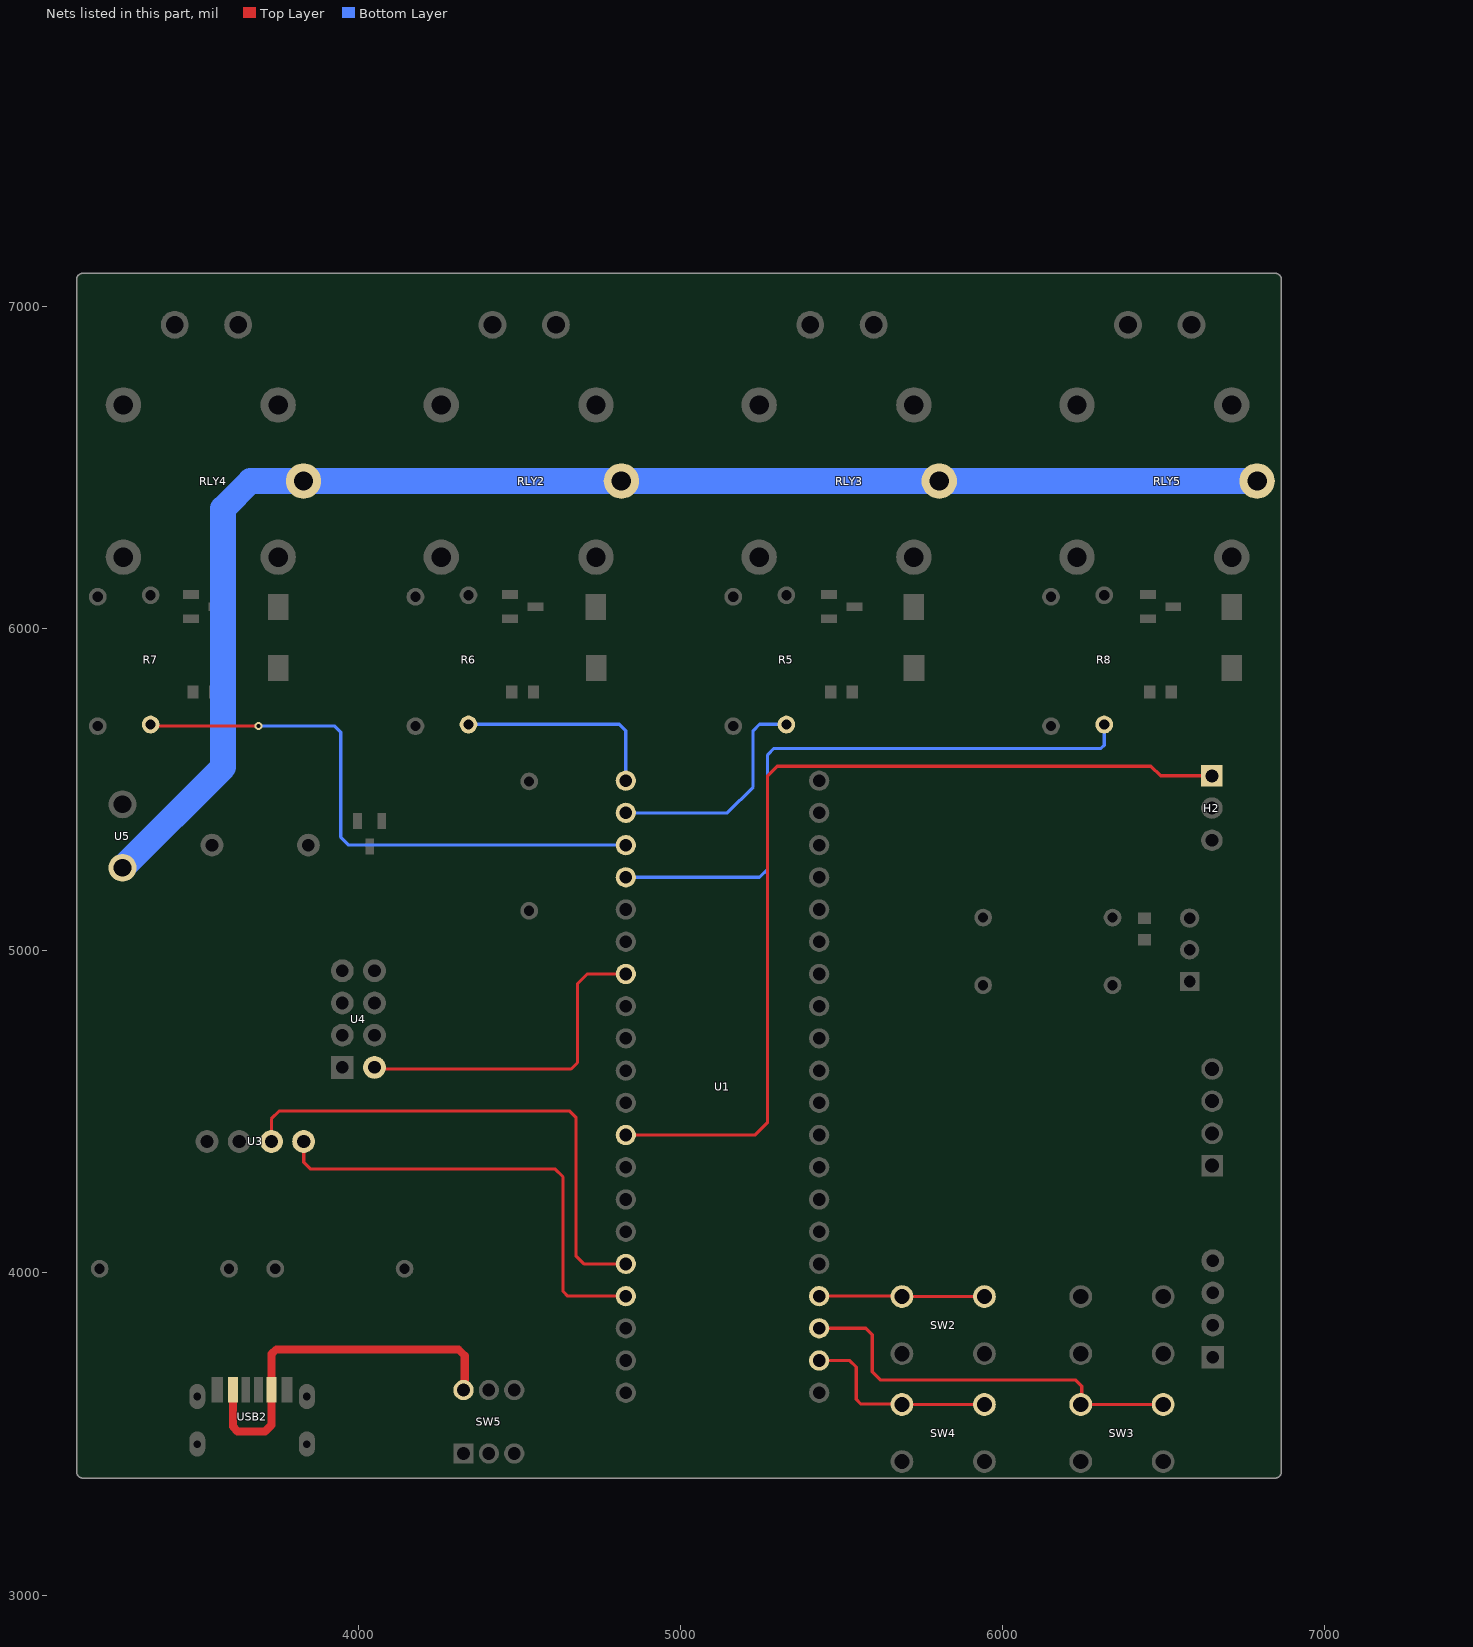
[diagram p0: the nets of this part, all layers, seen from the top]
# Altium PCB MISC62342.pcbdoc (part 2 of 2)
Units mil, origin at the board's own origin, x right, y up, seen from the top; angles counter-clockwise.
Board outline 3740 x 3740 mil, 2 copper layers (Top Layer, Bottom Layer), stack 62.206 mil thick; 50 components, 45 nets, 189 pads, 190 vias.

## Via types
v1: diameter 24.02, hole 12, Top Layer to Bottom Layer, 190 vias

## Nets (pads, with @x,y where several pads share a name; then routed paths per layer and width w, separated by ;. In a path a pad name is that pad's centre, name@x,y a point inside that pad or via, vN(x,y) a via of type N, cw(c..) or ccw(c..) an arc to the next point about the centre after c; other vN are vias at no path point) (continued)
PA10: U1.7 U4.5 | length 1047.8
  Top Layer w10: U4.5@4050,4638.19 4055,4633.19 4660,4633.19 4680,4653.19 4680,4898.19 4710,4928.19 U1.7@4830,4928.19
PB4: H2.1 U1.12 | length 2935.6
  Top Layer w10: U1.12@4830,4428.19 5230,4428.19 5270,4468.19 5270,5543.19 5300,5573.19 6460,5573.19 6490,5543.19 H2.1@6649.21,5543.19
PB8: U1.16 U3.3 | length 1629
  Top Layer w10: U3.3@3730,4408.19 3730,4478.19 3755,4503.19 4655,4503.19 4675,4483.19 4675,4053.19 4700,4028.18 U1.16@4830,4028.19
PB9: U1.17 U3.4 | length 1444.9
  Top Layer w10: U3.4@3830,4408.19 3830,4343.19 3850,4323.19 4610,4323.19 4635,4298.19 4635,3943.19 4650,3928.18 U1.17@4830,3928.19
PB12: R6.1 U1.1 | length 651.9
  Bottom Layer w10: R6.1@4341.67,5702.41 4342.46,5703.19 4810,5703.19 4830,5683.19 U1.1@4830,5528.19
PB13: R5.1 U1.2 | length 715.1
  Bottom Layer w10: U1.2@4830,5428.19 5145,5428.19 5225,5508.19 5225,5683.19 5245,5703.19 5327.54,5703.19 R5.1@5328.33,5702.41
PB14: R7.1 U1.3 | length 1820.4
  Top Layer w10: R7.1@3355,5702.41 3359.21,5698.19 v1(3690,5698.19)
  Bottom Layer w10: v1(3690,5698.19) 3925,5698.19 3945,5678.19 3945,5353.19 3970,5328.19 U1.3@4830,5328.19
PB15: R8.1 U1.4 | length 1927
  Bottom Layer w10: U1.4@4830,5228.19 5245,5228.19 5270,5253.19 5270,5608.19 5290,5628.19 6305,5628.19 6315,5638.19 R8.1@6315,5702.41
PC13: SW4.1 SW4.2 U1.22 | length 628
  Top Layer w10: U1.22@5430,3728.19 5525,3728.18 5545,3708.19 5545,3608.19 5560,3593.19 5665.63,3593.19 5667.05,3591.77 SW4.1@5687.05,3591.77 SW4.2@5942.95,3591.77
PC14: SW3.1 SW3.2 U1.23 | length 1270.5
  Top Layer w10: U1.23@5430,3828.19 5575,3828.18 5595,3808.19 5595,3693.19 5620,3668.19 6225,3668.19 6245,3648.19 6245,3594.72 SW3.1@6242.05,3591.77 SW3.2@6497.95,3591.77
PC15: SW2.1 SW2.2 U1.24 | length 513.5
  Top Layer w10: U1.24@5430,3928.19 5685.63,3928.18 SW2.1@5687.05,3926.77 SW2.2@5942.95,3926.77
VBUS: SW5.4 USB2.A9 USB2.B9 | length 1191.4
  Top Layer w25: USB2.B9@3610.16,3637.4 3610.16,3523.03 3625,3508.19 3710,3508.19 3730,3528.19 3730,3637.24 USB2.A9@3729.84,3637.4 3729.84,3748.03 3745,3763.19 4310,3763.19 4330,3743.19 4330,3640.35 SW5.4@4326.26,3636.62
VM: RLY2.5 RLY3.5 RLY4.5 RLY5.5 U5.2 | length 4489.5
  Bottom Layer w80: U5.2@3267.64,5257.86 3580,5570.22 3580,6373.19 3665,6458.19 RLY4.5@3829.53,6458.19 RLY2.5@4816.19,6458.19 RLY3.5@5802.86,6458.19 RLY5.5@6789.53,6458.19
pads on no net: H3.2 RLY2.3 RLY3.3 RLY4.3 RLY5.3 SW5.1 SW5.2 SW5.3 SW5.6 U1.8 U1.9 U1.10 U1.11 U1.13 U1.14 U1.15 U1.21 U1.30 U1.31 U1.32 U1.33 U1.34 U1.35 U1.36 U1.37 U4.2 U4.3 U4.6 U4.7
copper on no net:
  other v1: 3925,7773.19

## Polygon pours and split planes (outlines as drawn)
GND on Top Layer (solid, remove dead copper, pour order 0): 3055,7168.19 3055,3253.19 7025,3253.19 7025,7168.19
GND on Bottom Layer (solid, remove dead copper, pour order 2): 3000,7263.19 3000,3271.35 6985.25,3271.35 6985.25,7263.19

## Keep-outs
Board Outline Layer:
  region: 3130,5103.19 3130,4493.19 3460,4493.19 3460,5103.19
  region: 3136.57,6765.27 3136.57,6151.1 3892.49,6151.1 3892.49,6765.27
  region: 4123.24,6765.27 4123.24,6151.1 4879.15,6151.1 4879.15,6765.27
  region: 5109.9,6765.27 5109.9,6151.1 5865.82,6151.1 5865.82,6765.27
  region: 6096.57,6765.27 6096.57,6151.1 6852.49,6151.1 6852.49,6765.27
  lines w10: 3125,3383.19 3125,7083.19 cw(c3145,7083.19) 3145,7103.19 6845,7103.19 cw(c6845,7083.19) 6865,7083.19 6865,3383.19 cw(c6845,3383.19) 6845,3363.19 3145,3363.19 cw(c3145,3383.19) 3125,3383.19

## Other copper
Top Layer:
  region net +5V: 5736.99,5800.76 5711.99,5800.76 5711.68,5806.18 5710.74,5811.53 5709.19,5816.73 5707.04,5821.72 5704.34,5826.43 5701.11,5830.79 5697.39,5834.75 5693.24,5838.26 5755.74,5838.26 5751.59,5834.75 5747.88,5830.79 5744.65,5826.43 5741.94,5821.72 5739.8,5816.73 5738.25,5811.53 5737.31,5806.18 5736.99,5800.76
  region net +5V: 5793.88,5891.04 5793.88,5866.04 5788.46,5865.73 5783.11,5864.79 5777.91,5863.24 5772.92,5861.09 5768.21,5858.39 5763.85,5855.16 5759.89,5851.44 5756.38,5847.29 5756.38,5909.79 5759.89,5905.64 5763.85,5901.93 5768.21,5898.7 5772.92,5895.99 5777.91,5893.85 5783.11,5892.3 5788.46,5891.36 5793.88,5891.04
  region net +5V: 5655.1,5866.04 5655.1,5891.04 5660.52,5891.36 5665.87,5892.3 5671.08,5893.85 5676.07,5895.99 5680.77,5898.7 5685.14,5901.93 5689.1,5905.64 5692.6,5909.79 5692.6,5847.29 5689.1,5851.44 5685.14,5855.16 5680.77,5858.39 5676.07,5861.09 5671.08,5863.24 5665.87,5864.79 5660.52,5865.73 5655.1,5866.04
  region net +5V: 4773.69,5932.08 4782.97,5906.01 4779.02,5900.11 4775.72,5893.81 4773.12,5887.2 4771.23,5880.35 4770.1,5873.33 4769.72,5866.24 4733.91,5918.82 4741.01,5919.21 4748.03,5920.34 4754.88,5922.23 4761.49,5924.83 4767.78,5928.13 4773.69,5932.08
  region net +5V: 4807.22,5890.69 4807.22,5865.69 4801.79,5865.37 4796.45,5864.43 4791.24,5862.88 4786.25,5860.74 4781.54,5858.03 4777.18,5854.8 4773.22,5851.09 4769.72,5846.94 4769.72,5909.44 4773.22,5905.29 4777.18,5901.57 4781.54,5898.34 4786.25,5895.64 4791.24,5893.49 4796.45,5891.94 4801.79,5891 4807.22,5890.69
  region net +5V: 4752.5,5800.76 4727.5,5800.76 4727.19,5806.18 4726.25,5811.53 4724.69,5816.73 4722.55,5821.72 4719.85,5826.43 4716.61,5830.79 4712.9,5834.75 4708.75,5838.26 4769.72,5838.26 4765.36,5834.02 4761.56,5829.28 4758.36,5824.11 4755.83,5818.59 4753.99,5812.8 4752.87,5806.82 4752.5,5800.76
  region net +5V: 3762.5,5800.76 3737.5,5800.76 3737.1,5806.91 3735.91,5812.95 3733.96,5818.79 3731.26,5824.33 3727.88,5829.48 3723.86,5834.15 3719.27,5838.26 3781.25,5838.26 3777.1,5834.75 3773.39,5830.79 3770.15,5826.43 3767.45,5821.72 3765.31,5816.73 3763.75,5811.53 3762.81,5806.18 3762.5,5800.76
  region net +5V: 3820.55,5885.69 3820.55,5860.69 3815.13,5860.37 3809.78,5859.43 3804.58,5857.88 3799.59,5855.74 3794.88,5853.03 3790.51,5849.8 3786.55,5846.09 3783.05,5841.94 3783.05,5904.44 3786.55,5900.29 3790.51,5896.57 3794.88,5893.34 3799.59,5890.64 3804.58,5888.49 3809.78,5886.94 3815.13,5886 3820.55,5885.69
  region net +5V: 3787.02,5932.08 3796.31,5906.01 3792.35,5900.11 3789.06,5893.81 3786.45,5887.2 3784.57,5880.35 3783.43,5873.33 3783.05,5866.24 3747.25,5918.82 3754.34,5919.21 3761.36,5920.34 3768.21,5922.23 3774.82,5924.83 3781.12,5928.13 3787.02,5932.08
  region net +5V: 6756.31,5851.07 6747.02,5825 6741.12,5828.95 6734.82,5832.25 6728.21,5834.86 6721.36,5836.74 6714.34,5837.88 6707.25,5838.26 6743.05,5890.85 6743.43,5883.75 6744.57,5876.74 6746.45,5869.88 6749.06,5863.27 6752.35,5856.98 6756.31,5851.07
  region net +5V: 6747.02,5932.08 6756.31,5906.01 6752.35,5900.11 6749.06,5893.81 6746.45,5887.2 6744.57,5880.35 6743.43,5873.33 6743.05,5866.24 6707.25,5918.82 6714.34,5919.21 6721.36,5920.34 6728.21,5922.23 6734.82,5924.83 6741.12,5928.13 6747.02,5932.08
  region net PB4: 6600.75,5538.19 6600.75,5548.19 6604.2,5548.51 6607.54,5549.46 6610.65,5551.02 6613.42,5553.11 6615.75,5555.69 6615.75,5530.69 6613.42,5533.26 6610.65,5535.36 6607.54,5536.91 6604.2,5537.87 6600.75,5538.19
  region net +5V: 6694.77,5455.69 6694.77,5430.69 6691.32,5430.4 6688.1,5429.6 6685.06,5428.36 6682.17,5426.75 6679.39,5424.84 6676.68,5422.71 6671.35,5418.09 6671.35,5468.29 6676.68,5463.66 6679.39,5461.53 6682.17,5459.62 6685.06,5458.01 6688.1,5456.77 6691.32,5455.97
  region net +3.3V: 6645,4682.25 6665,4674.75 6665.08,4672.6 6665.29,4670.68 6665.65,4668.96 6666.13,4667.41 6666.72,4666 6667.42,4664.7 6669.1,4662.31 6673.3,4657.57 6675.68,4654.75 6678.12,4651.32 6628.49,4658.82 6634.55,4663.89 6637.34,4666.44 6639.84,4669.09 6641.95,4671.93 6642.83,4673.44 6643.58,4675.02 6644.18,4676.68 6644.63,4678.43 6644.91,4680.29
  region net +3.3V: 6691.56,4648.19 6699.06,4628.19 6697.1,4628.09 6695.25,4627.82 6693.49,4627.37 6691.83,4626.77 6690.25,4626.02 6688.74,4625.14 6685.91,4623.03 6683.25,4620.53 6680.7,4617.74 6675.64,4611.68 6668.14,4661.31 6671.57,4658.86 6674.39,4656.49 6679.12,4652.29 6681.51,4650.61 6682.81,4649.91 6684.22,4649.31 6685.78,4648.84 6687.5,4648.48 6689.41,4648.26
  region net +5V: 4189.52,5659.88 4164.52,5659.88 4164.33,5662.29 4163.81,5664.85 4163.01,5667.47 4161.96,5670.1 4160.73,5672.66 4159.35,5675.07 4157.87,5677.26 4156.35,5679.17 4197.69,5679.17 4196.16,5677.26 4194.69,5675.07 4193.31,5672.66 4192.07,5670.1 4191.02,5667.47 4190.22,5664.85 4189.7,5662.29
  region net +5V: 4139.5,5684.9 4139.5,5709.9 4141.91,5710.08 4144.46,5710.6 4147.09,5711.4 4149.72,5712.45 4152.28,5713.69 4154.69,5715.07 4156.88,5716.54 4158.79,5718.07 4158.79,5676.73 4156.88,5678.25 4154.69,5679.73 4152.28,5681.11 4149.72,5682.34 4147.09,5683.39 4144.46,5684.19 4141.91,5684.71
  region net +5V: 5198.74,5679.71 5181.06,5662.03 5179.23,5663.6 5177.05,5665.04 5174.62,5666.33 5172.03,5667.45 5169.34,5668.39 5166.66,5669.11 5164.07,5669.62 5161.64,5669.89 5190.87,5699.12 5191.14,5696.7 5191.65,5694.1 5192.38,5691.42 5193.31,5688.74 5194.43,5686.14 5195.72,5683.71 5197.16,5681.54
  region net +5V: 5125.85,5684.9 5125.85,5709.9 5128.26,5710.08 5130.82,5710.6 5133.45,5711.4 5136.07,5712.45 5138.63,5713.69 5141.04,5715.07 5143.23,5716.54 5145.14,5718.07 5145.14,5676.73 5143.23,5678.25 5141.04,5679.73 5138.63,5681.11 5136.07,5682.34 5133.45,5683.39 5130.82,5684.19 5128.26,5684.71
  region net +5V: 3203.16,5659.88 3178.16,5659.88 3177.98,5662.29 3177.46,5664.85 3176.66,5667.47 3175.61,5670.1 3174.37,5672.66 3172.99,5675.07 3171.52,5677.26 3169.99,5679.17 3211.33,5679.17 3209.81,5677.26 3208.33,5675.07 3206.95,5672.66 3205.72,5670.1 3204.67,5667.47 3203.87,5664.85 3203.35,5662.29
  region net +5V: 6115.57,5680.69 6109.26,5705.69 6111.67,5705.9 6114.29,5706.49 6117.01,5707.41 6119.72,5708.61 6122.34,5710.03 6124.75,5711.61 6126.85,5713.29 6128.55,5715.04 6134.86,5674.19 6130.56,5676.57 6128.12,5677.67 6125.57,5678.66 6122.99,5679.49 6120.42,5680.13 6117.92,5680.54
  region net PA8: 4567.52,5129.25 4567.52,5119.25 4565.45,5119.16 4563.65,5118.9 4562.1,5118.47 4560.76,5117.9 4559.59,5117.19 4558.55,5116.36 4556.76,5114.35 4553.32,5109.33 4551.12,5106.5 4549.78,5105.05 4548.23,5103.58 4548.23,5144.92 4549.78,5143.45 4551.12,5141.99 4553.32,5139.16 4556.76,5134.14 4558.55,5132.14 4559.59,5131.3 4560.76,5130.59 4562.1,5130.02 4563.65,5129.6 4565.45,5129.34
  region net PA3: 6350,4859.04 6340,4852.72 6339.9,4854.67 6339.62,4856.41 6339.17,4857.98 6338.55,4859.38 6337.79,4860.64 6336.89,4861.8 6334.73,4863.85 6332.18,4865.72 6329.34,4867.58 6326.29,4869.62 6323.15,4872.01 6364,4878.33 6362.39,4876.2 6360.34,4873.92 6355.69,4869.07 6353.51,4866.55 6351.7,4864.02 6350.99,4862.76 6350.46,4861.51 6350.12,4860.27
  region net PA3: 6378.31,4898.19 6378.31,4888.19 6376.24,4888.1 6374.44,4887.84 6372.89,4887.41 6371.55,4886.84 6370.38,4886.13 6369.34,4885.29 6367.55,4883.29 6364.11,4878.27 6361.91,4875.44 6360.57,4873.98 6359.02,4872.52 6359.02,4913.86 6360.57,4912.39 6361.91,4910.93 6364.11,4908.1 6367.55,4903.08 6369.34,4901.08 6370.38,4900.24 6371.55,4899.53 6372.89,4898.96 6374.44,4898.54 6376.24,4898.28
  region net +3.3V: 5929.21,4930.71 5949.21,4930.71 5949.45,4927.81 5950.13,4925.14 5951.18,4922.65 5952.54,4920.31 5954.16,4918.05 5955.96,4915.85 5959.88,4911.42 5918.54,4911.42 5922.46,4915.85 5924.26,4918.05 5925.88,4920.31 5927.24,4922.65 5928.29,4925.14 5928.97,4927.81
  region net +3.3V: 5949.21,5065.67 5929.21,5065.67 5928.97,5068.56 5928.29,5071.23 5927.24,5073.72 5925.88,5076.07 5924.26,5078.32 5922.46,5080.53 5918.54,5084.96 5959.88,5084.96 5955.96,5080.53 5954.16,5078.32 5952.54,5076.07 5951.18,5073.72 5950.13,5071.23 5949.45,5068.56
  region net +5V: 4800.06,6230.81 4821.52,6173.98 4819.01,6176.32 4816.32,6178.47 4813.49,6180.41 4810.53,6182.14 4807.47,6183.65 4804.32,6184.9 4801.12,6185.89 4797.89,6186.61 4794.65,6187.03 4791.42,6187.15 4788.23,6186.94 4785.1,6186.4 4782.05,6185.5 4779.11,6184.23 4776.29,6182.59 4773.63,6180.54 4774.74,6262.4 4779.52,6257.69 4782.96,6253.69 4785.52,6250.15 4787.61,6246.82 4789.68,6243.47 4792.16,6239.85 4795.47,6235.71
  region net +5V: 5798.08,6235.69 5799.91,6210.69 5796.11,6210.52 5792.73,6210.03 5789.72,6209.25 5787.04,6208.18 5784.63,6206.86 5782.44,6205.31 5780.42,6203.54 5778.52,6201.58 5774.87,6197.16 5771.07,6192.24 5766.72,6186.97 5764.21,6184.26 5761.41,6181.53 5759.58,6264.01 5762.54,6261.36 5765.15,6258.73 5769.59,6253.61 5773.35,6248.83 5776.89,6244.54 5778.72,6242.63 5780.67,6240.92 5782.8,6239.4 5785.16,6238.12 5787.81,6237.09 5790.81,6236.32 5794.21,6235.85
  region net +5V: 3825.67,6234.47 3825.67,6209.47 3821.83,6209.3 3818.44,6208.82 3815.44,6208.05 3812.78,6207 3810.39,6205.7 3808.23,6204.16 3806.25,6202.42 3804.38,6200.48 3800.78,6196.13 3797.01,6191.27 3792.61,6186.08 3790.05,6183.41 3787.17,6180.72 3787.17,6263.22 3790.05,6260.53 3792.61,6257.86 3797.01,6252.66 3800.78,6247.8 3804.38,6243.45 3806.25,6241.52 3808.23,6239.77 3810.39,6238.24 3812.78,6236.94 3815.44,6235.89 3818.44,6235.11 3821.83,6234.63
  region net +5V: 6774.23,6196.64 6771.87,6163.64 6769.27,6165.98 6766.58,6167.9 6763.81,6169.44 6760.97,6170.63 6758.04,6171.49 6755.04,6172.06 6751.98,6172.37 6748.85,6172.44 6745.65,6172.3 6742.4,6171.99 6735.74,6170.96 6721.88,6168.1 6762.85,6239.71 6763.55,6237.34 6764.15,6234.78 6765.09,6229.17 6766.71,6217.03 6767.76,6211.04 6768.43,6208.19 6769.24,6205.47 6770.19,6202.92 6771.33,6200.57 6772.66,6198.47
  region net PA0: 6237.05,3975.01 6247.05,3975.01 6247.17,3972.18 6247.53,3969.76 6248.12,3967.71 6248.9,3965.97 6249.88,3964.49 6251.03,3963.22 6252.34,3962.1 6253.79,3961.08 6260.7,3956.95 6262.63,3955.64 6264.6,3954.11 6266.6,3952.32 6268.62,3950.2 6215.48,3950.2 6217.5,3952.32 6219.5,3954.11 6221.47,3955.64 6223.4,3956.95 6230.31,3961.08 6231.76,3962.1 6233.07,3963.22 6234.22,3964.49 6235.2,3965.97 6235.98,3967.71 6236.57,3969.76 6236.93,3972.18
  region net PA0: 6290.29,3931.77 6290.29,3921.77 6287.46,3921.64 6285.04,3921.28 6282.99,3920.7 6281.25,3919.91 6279.77,3918.94 6278.5,3917.78 6277.38,3916.48 6276.36,3915.02 6272.23,3908.11 6270.92,3906.19 6269.4,3904.22 6267.6,3902.21 6265.49,3900.19 6265.49,3953.34 6267.6,3951.32 6269.4,3949.32 6270.92,3947.34 6272.23,3945.42 6276.36,3938.51 6277.38,3937.06 6278.5,3935.75 6279.77,3934.6 6281.25,3933.62 6282.99,3932.83 6285.04,3932.25 6287.46,3931.89
  region net PA0: 6449.71,3921.77 6449.71,3931.77 6452.54,3931.89 6454.96,3932.25 6457.01,3932.83 6458.75,3933.62 6460.23,3934.6 6461.5,3935.75 6462.62,3937.06 6463.64,3938.51 6467.77,3945.42 6469.08,3947.34 6470.6,3949.32 6472.4,3951.32 6474.51,3953.34 6474.51,3900.19 6472.4,3902.21 6470.6,3904.22 6469.08,3906.19 6467.77,3908.11 6463.64,3915.02 6462.62,3916.48 6461.5,3917.78 6460.23,3918.94 6458.75,3919.91 6457.01,3920.7 6454.96,3921.28 6452.54,3921.64
  region net PC15: 5637.77,3923.18 5639.89,3933.18 5641.48,3933.36 5643.09,3933.87 5644.73,3934.68 5646.38,3935.74 5649.7,3938.46 5653,3941.75 5659.26,3948.74 5662.11,3951.84 5664.7,3954.26 5662.57,3901.15 5660.57,3903.21 5658.85,3905.26 5656.07,3909.24 5653.86,3912.96 5651.82,3916.3 5650.75,3917.78 5649.58,3919.12 5648.26,3920.29 5646.75,3921.29 5644.99,3922.1 5642.94,3922.69 5640.55,3923.06
  region net PC15: 5735.29,3931.77 5735.29,3921.77 5732.46,3921.64 5730.04,3921.28 5727.99,3920.7 5726.25,3919.91 5724.77,3918.94 5723.5,3917.78 5722.38,3916.48 5721.36,3915.02 5717.23,3908.11 5715.92,3906.19 5714.4,3904.22 5712.6,3902.21 5710.49,3900.19 5710.49,3953.34 5712.6,3951.32 5714.4,3949.32 5715.92,3947.34 5717.23,3945.42 5721.36,3938.51 5722.38,3937.06 5723.5,3935.75 5724.77,3934.6 5726.25,3933.62 5727.99,3932.83 5730.04,3932.25 5732.46,3931.89
  region net PC15: 5894.71,3921.77 5894.71,3931.77 5897.54,3931.89 5899.96,3932.25 5902.01,3932.83 5903.75,3933.62 5905.23,3934.6 5906.5,3935.75 5907.62,3937.06 5908.64,3938.51 5912.77,3945.42 5914.08,3947.34 5915.6,3949.32 5917.4,3951.32 5919.51,3953.34 5919.51,3900.19 5917.4,3902.21 5915.6,3904.22 5914.08,3906.19 5912.77,3908.11 5908.64,3915.02 5907.62,3916.48 5906.5,3917.78 5905.23,3918.94 5903.75,3919.91 5902.01,3920.7 5899.96,3921.28 5897.54,3921.64
  region net PC14: 6240,3642.14 6250,3637.71 6250.17,3636.1 6250.67,3634.47 6251.45,3632.83 6252.48,3631.19 6255.13,3627.91 6258.32,3624.68 6265.12,3618.48 6268.13,3615.6 6270.48,3612.91 6217.52,3617.33 6219.62,3619.22 6221.71,3620.86 6225.77,3623.57 6229.57,3625.81 6232.97,3627.94 6234.49,3629.06 6235.85,3630.29 6237.05,3631.65 6238.07,3633.21 6238.89,3634.99 6239.5,3637.04 6239.87,3639.41
  region net PC14: 6290.29,3596.77 6290.29,3586.77 6287.46,3586.64 6285.04,3586.28 6282.99,3585.7 6281.25,3584.91 6279.77,3583.94 6278.5,3582.78 6277.38,3581.48 6276.36,3580.02 6272.23,3573.11 6270.92,3571.19 6269.4,3569.22 6267.6,3567.21 6265.49,3565.19 6265.49,3618.34 6267.6,3616.32 6269.4,3614.32 6270.92,3612.34 6272.23,3610.42 6276.36,3603.51 6277.38,3602.06 6278.5,3600.75 6279.77,3599.6 6281.25,3598.62 6282.99,3597.83 6285.04,3597.25 6287.46,3596.89
  region net PC14: 6449.71,3586.77 6449.71,3596.77 6452.54,3596.89 6454.96,3597.25 6457.01,3597.83 6458.75,3598.62 6460.23,3599.6 6461.5,3600.75 6462.62,3602.06 6463.64,3603.51 6467.77,3610.42 6469.08,3612.34 6470.6,3614.32 6472.4,3616.32 6474.51,3618.34 6474.51,3565.19 6472.4,3567.21 6470.6,3569.22 6469.08,3571.19 6467.77,3573.11 6463.64,3580.02 6462.62,3581.48 6461.5,3582.78 6460.23,3583.94 6458.75,3584.91 6457.01,3585.7 6454.96,3586.28 6452.54,3586.64
  region net PC13: 5735.29,3596.77 5735.29,3586.77 5732.46,3586.64 5730.04,3586.28 5727.99,3585.7 5726.25,3584.91 5724.77,3583.94 5723.5,3582.78 5722.38,3581.48 5721.36,3580.02 5717.23,3573.11 5715.92,3571.19 5714.4,3569.22 5712.6,3567.21 5710.49,3565.19 5710.49,3618.34 5712.6,3616.32 5714.4,3614.32 5715.92,3612.34 5717.23,3610.42 5721.36,3603.51 5722.38,3602.06 5723.5,3600.75 5724.77,3599.6 5726.25,3598.62 5727.99,3597.83 5730.04,3597.25 5732.46,3596.89
  region net PC13: 5637.76,3588.19 5639.89,3598.19 5641.48,3598.37 5643.09,3598.88 5644.73,3599.68 5646.38,3600.74 5649.7,3603.47 5653,3606.75 5659.26,3613.74 5662.11,3616.84 5664.7,3619.26 5662.57,3566.15 5660.56,3568.22 5658.85,3570.26 5656.07,3574.24 5653.86,3577.97 5651.82,3581.3 5650.75,3582.78 5649.58,3584.12 5648.26,3585.3 5646.75,3586.29 5644.99,3587.1 5642.93,3587.69 5640.54,3588.06
  region net PC13: 5894.71,3586.77 5894.71,3596.77 5897.54,3596.89 5899.96,3597.25 5902.01,3597.83 5903.75,3598.62 5905.23,3599.6 5906.5,3600.75 5907.62,3602.06 5908.64,3603.51 5912.77,3610.42 5914.08,3612.34 5915.6,3614.32 5917.4,3616.32 5919.51,3618.34 5919.51,3565.19 5917.4,3567.21 5915.6,3569.22 5914.08,3571.19 5912.77,3573.11 5908.64,3580.02 5907.62,3581.48 5906.5,3582.78 5905.23,3583.94 5903.75,3584.91 5902.01,3585.7 5899.96,3586.28 5897.54,3586.64
  region net VBUS: 4317.5,3682.15 4342.5,3676.54 4342.72,3673.43 4343.33,3670.48 4344.29,3667.67 4345.53,3664.95 4346.99,3662.31 4348.63,3659.7 4352.19,3654.49 4305.28,3660.1 4307.56,3662.28 4309.77,3664.7 4311.83,3667.31 4313.68,3670.1 4315.24,3673.01 4316.45,3676.01 4317.23,3679.07
  region net +5V: 4392.5,3679.49 4417.5,3679.49 4417.75,3676.39 4418.46,3673.39 4419.56,3670.48 4420.98,3667.68 4422.66,3664.97 4424.54,3662.37 4428.62,3657.44 4381.38,3657.44 4385.46,3662.37 4387.34,3664.97 4389.03,3667.68 4390.45,3670.48 4391.55,3673.39 4392.25,3676.39
  region net PA2: 6603.73,3933.19 6603.73,3943.19 6606.56,3943.31 6608.98,3943.67 6611.03,3944.25 6612.76,3945.04 6614.24,3946.02 6615.52,3947.17 6616.64,3948.48 6617.66,3949.93 6621.79,3956.84 6623.1,3958.76 6624.62,3960.74 6626.42,3962.74 6628.53,3964.76 6628.53,3911.61 6626.42,3913.63 6624.62,3915.64 6623.1,3917.61 6621.79,3919.53 6617.66,3926.44 6616.64,3927.9 6615.52,3929.2 6614.24,3930.36 6612.76,3931.33 6611.03,3932.12 6608.98,3932.7 6606.56,3933.06
  region net +3.3V: 6717.4,3748.19 6717.4,3728.19 6712.45,3727.86 6707.58,3726.88 6702.89,3725.26 6698.45,3723.04 6694.34,3720.26 6690.64,3716.95 6687.4,3713.19 6687.4,3763.19 6690.64,3759.42 6694.34,3756.12 6698.45,3753.33 6702.89,3751.11 6707.58,3749.5 6712.45,3748.52 6717.4,3748.19
  region net +3.3V: 3625,4459.94 3645,4452.44 3645.08,4450.09 3645.33,4448.01 3645.72,4446.16 3646.26,4444.52 3646.92,4443.03 3647.7,4441.68 3649.57,4439.22 3654.25,4434.34 3656.89,4431.35 3659.62,4427.64 3607,4435.14 3613.61,4440.59 3616.65,4443.24 3619.37,4445.98 3621.68,4448.92 3622.64,4450.49 3623.45,4452.15 3624.11,4453.92 3624.6,4455.79 3624.9,4457.8
  region net PB8: 3725,4456.43 3735,4456.43 3735.12,4453.6 3735.48,4451.18 3736.07,4449.13 3736.85,4447.39 3737.83,4445.91 3738.98,4444.64 3740.29,4443.52 3741.74,4442.5 3748.65,4438.37 3750.58,4437.06 3752.55,4435.53 3754.55,4433.74 3756.57,4431.62 3703.43,4431.62 3705.45,4433.74 3707.45,4435.53 3709.42,4437.06 3711.35,4438.37 3718.26,4442.5 3719.71,4443.52 3721.02,4444.64 3722.17,4445.91 3723.15,4447.39 3723.93,4449.13 3724.52,4451.18 3724.88,4453.6
  region net PB9: 3835,4359.95 3825,4359.95 3824.88,4362.78 3824.52,4365.19 3823.93,4367.24 3823.15,4368.98 3822.17,4370.46 3821.02,4371.74 3819.71,4372.86 3818.26,4373.88 3811.35,4378.01 3809.42,4379.32 3807.45,4380.84 3805.45,4382.64 3803.43,4384.75 3856.57,4384.75 3854.55,4382.64 3852.55,4380.84 3850.58,4379.32 3848.65,4378.01 3841.74,4373.88 3840.29,4372.86 3838.98,4371.74 3837.83,4370.46 3836.85,4368.98 3836.07,4367.24 3835.48,4365.19 3835.12,4362.78
  region net PA10: 4101.76,4638.19 4094.26,4628.19 4092.59,4628.02 4090.93,4627.55 4089.29,4626.8 4087.66,4625.81 4084.45,4623.27 4081.3,4620.22 4075.22,4613.7 4072.3,4610.82 4069.45,4608.57 4076.95,4661.19 4078.68,4659.04 4080.22,4656.9 4082.84,4652.74 4085.13,4648.86 4087.36,4645.38 4088.56,4643.83 4089.85,4642.43 4091.28,4641.21 4092.88,4640.16 4094.69,4639.32 4096.75,4638.7 4099.09,4638.32
  region net PA9: 3945,4986.43 3955,4986.43 3955.12,4983.6 3955.48,4981.18 3956.07,4979.13 3956.85,4977.39 3957.83,4975.91 3958.98,4974.64 3960.29,4973.52 3961.74,4972.5 3968.65,4968.37 3970.58,4967.06 3972.55,4965.53 3974.55,4963.74 3976.57,4961.62 3923.43,4961.62 3925.45,4963.74 3927.45,4965.53 3929.42,4967.06 3931.35,4968.37 3938.26,4972.5 3939.71,4973.52 3941.02,4974.64 3942.17,4975.91 3943.15,4977.39 3943.93,4979.13 3944.52,4981.18 3944.88,4983.6
  region net +3.3V: 6638.43,4914.76 6638.43,4894.76 6633.66,4894.43 6628.99,4893.44 6624.5,4891.82 6620.28,4889.59 6616.41,4886.8 6612.96,4883.51 6610,4879.76 6610,4929.76 6612.96,4926.02 6616.41,4922.72 6620.28,4919.93 6624.5,4917.7 6628.99,4916.08 6633.66,4915.09 6638.43,4914.76
  region net PA3: 6539.15,4998.19 6539.16,5008.19 6541.47,5008.29 6543.45,5008.58 6545.16,5009.05 6546.63,5009.69 6547.89,5010.48 6549,5011.42 6550.9,5013.66 6554.55,5019.26 6556.95,5022.42 6558.43,5024.05 6560.16,5025.69 6560.15,4980.69 6558.43,4982.32 6556.95,4983.95 6554.55,4987.11 6550.89,4992.72 6549,4994.96 6547.89,4995.89 6546.62,4996.68 6545.15,4997.32 6543.45,4997.79 6541.46,4998.09
  region net VBUS: 3622.66,3576.28 3597.66,3576.28 3597.3,3588.84 3596.21,3601.35 3594.41,3613.78 3625.91,3613.78 3624.11,3601.35 3623.02,3588.84 3622.66,3576.28
  region net VBUS: 3717.34,3698.52 3742.34,3698.52 3742.7,3685.97 3743.79,3673.45 3745.59,3661.02 3714.09,3661.02 3715.89,3673.45 3716.98,3685.97 3717.34,3698.52
  region net VBUS: 3742.5,3576.28 3717.5,3576.28 3717.12,3588.84 3715.98,3601.36 3714.09,3613.78 3745.59,3613.78 3743.87,3601.34 3742.84,3588.83 3742.5,3576.28
Bottom Layer:
  region net +5V: 6600.15,5435.69 6607.65,5460.69 6611.13,5460.93 6614.29,5461.6 6617.2,5462.65 6619.95,5464.01 6622.63,5465.61 6625.32,5467.41 6631.08,5471.31 6623.58,5421.68 6621.26,5424.29 6618.72,5426.82 6615.99,5429.19 6613.09,5431.31 6610.03,5433.1 6606.84,5434.48 6603.54,5435.37 6601.86,5435.61
  region net PA4: 6601.54,4323.19 6601.54,4333.19 6604.99,4333.51 6608.33,4334.46 6611.44,4336.02 6614.2,4338.11 6616.54,4340.69 6616.54,4315.69 6614.2,4318.26 6611.44,4320.36 6608.33,4321.91 6604.99,4322.87 6601.54,4323.19
  region net PB13: 5290.23,5698.19 5291.41,5708.19 5293.51,5708.28 5295.32,5708.53 5296.87,5708.95 5298.2,5709.51 5299.36,5710.21 5300.37,5711.03 5302.1,5713 5305.48,5717.93 5307.71,5720.71 5309.1,5722.14 5310.7,5723.58 5309.52,5682.26 5306.72,5685.23 5304.55,5688.11 5302.75,5690.8 5301.05,5693.21 5299.21,5695.25 5298.16,5696.1 5296.97,5696.82 5295.61,5697.4 5294.06,5697.83 5292.27,5698.1
  region net PB12: 4378.59,5708.19 4379.77,5698.19 4377.73,5698.1 4375.94,5697.83 4374.39,5697.4 4373.03,5696.82 4371.84,5696.1 4370.79,5695.25 4368.95,5693.21 4367.25,5690.8 4365.45,5688.11 4363.28,5685.23 4360.48,5682.26 4359.3,5723.58 4360.9,5722.14 4362.29,5720.71 4364.52,5717.93 4367.9,5713 4369.63,5711.03 4370.64,5710.21 4371.8,5709.51 4373.13,5708.95 4374.68,5708.53 4376.49,5708.28
  region net +3.3V: 5949.21,4855.67 5929.21,4855.67 5928.97,4858.56 5928.29,4861.23 5927.24,4863.72 5925.88,4866.07 5924.26,4868.32 5922.46,4870.53 5918.54,4874.96 5959.88,4874.96 5955.96,4870.53 5954.16,4868.32 5952.54,4866.07 5951.18,4863.72 5950.13,4861.23 5949.45,4858.56
  region net PA1: 6603.73,3833.19 6603.73,3843.19 6606.56,3843.31 6608.98,3843.67 6611.03,3844.25 6612.76,3845.04 6614.24,3846.02 6615.52,3847.17 6616.64,3848.48 6617.66,3849.93 6621.79,3856.84 6623.1,3858.76 6624.62,3860.74 6626.42,3862.74 6628.53,3864.76 6628.53,3811.61 6626.42,3813.63 6624.62,3815.64 6623.1,3817.61 6621.79,3819.53 6617.66,3826.44 6616.64,3827.9 6615.52,3829.2 6614.24,3830.36 6612.76,3831.33 6611.03,3832.12 6608.98,3832.7 6606.56,3833.06
  region net +3.3V: 3640,4359.95 3620,4359.95 3619.9,4362.19 3619.63,4364.22 3619.18,4366.08 3618.58,4367.79 3617.82,4369.36 3616.94,4370.82 3614.82,4373.52 3612.31,4376.08 3609.51,4378.67 3606.52,4381.5 3603.43,4384.75 3656.57,4384.75 3653.48,4381.5 3650.49,4378.67 3647.69,4376.08 3645.18,4373.52 3643.06,4370.82 3642.18,4369.36 3641.42,4367.79 3640.82,4366.08 3640.37,4364.22 3640.1,4362.19
  region net +3.3V: 4040,4986.43 4060,4986.43 4060.1,4984.19 4060.37,4982.15 4060.82,4980.29 4061.42,4978.59 4062.18,4977.01 4063.06,4975.55 4065.18,4972.85 4067.69,4970.3 4070.49,4967.7 4073.48,4964.87 4076.57,4961.62 4023.43,4961.62 4026.52,4964.87 4029.51,4967.7 4032.31,4970.3 4034.82,4972.85 4036.94,4975.55 4037.82,4977.01 4038.58,4978.59 4039.18,4980.29 4039.63,4982.15 4039.9,4984.19
  region net +3.3V: 6590,4844.76 6570,4844.76 6569.67,4849.72 6568.69,4854.58 6567.08,4859.28 6564.86,4863.72 6562.07,4867.82 6558.77,4871.53 6555,4874.76 6605,4874.76 6601.23,4871.53 6597.93,4867.82 6595.14,4863.72 6592.92,4859.28 6591.31,4854.58 6590.33,4849.72 6590,4844.76

## Silkscreen, mask and mechanical layers (free items; w line width, h text height)
Top Silkscreen Layer:
  text "+" at 3234.97,6883.19 h120
  text "+" at 4221.64,6883.19 h120
  text "+" at 5208.3,6883.19 h120
  text "+" at 6194.97,6883.19 h120
  text "Add water" at 4743.91,6823.69 h120
  text "Heat" at 6708.91,6823.69 h120
  text "Drain water" at 5727.05,6819.69 h120
  text "Filter" at 3760,6818.24 h120
  text "1kΩ" at 3385.55,5846.37 h60 r90
  text "1kΩ" at 4372.21,5846.37 h60 r90
  text "1kΩ" at 5358.88,5846.37 h60 r90
  text "1kΩ" at 6345.55,5846.37 h60 r90
  text "10kΩ" at 3220.94,5824.38 h60 r90
  text "10kΩ" at 4207.29,5824.38 h60 r90
  text "10kΩ" at 5193.64,5824.38 h60 r90
  text "10kΩ" at 6179.99,5824.38 h60 r90
  text "PB4" at 6460,5513.1 h60
  text "1kΩ" at 4560,5265.04 h60 r90
  text "1kΩ" at 6080,5073.19 h60
  text "10kΩ" at 6080,4863.19 h60
  text "PA4" at 6460,4303.1 h60
  text "5.1kΩ" at 3312.88,3982.91 h60
  text "5.1kΩ" at 3857.76,3982.91 h60
  text "Switch page" at 6251.69,3983.19 h60
  text "Add/Confirm" at 5709.83,3982.1 h60
  text "Decrease" at 6339.95,3633.19 h60
  text "Select" at 5754.4,3630.46 h60

## Dimensions
3125,3363.19 to 6865.16,3363.19 on Document Layer